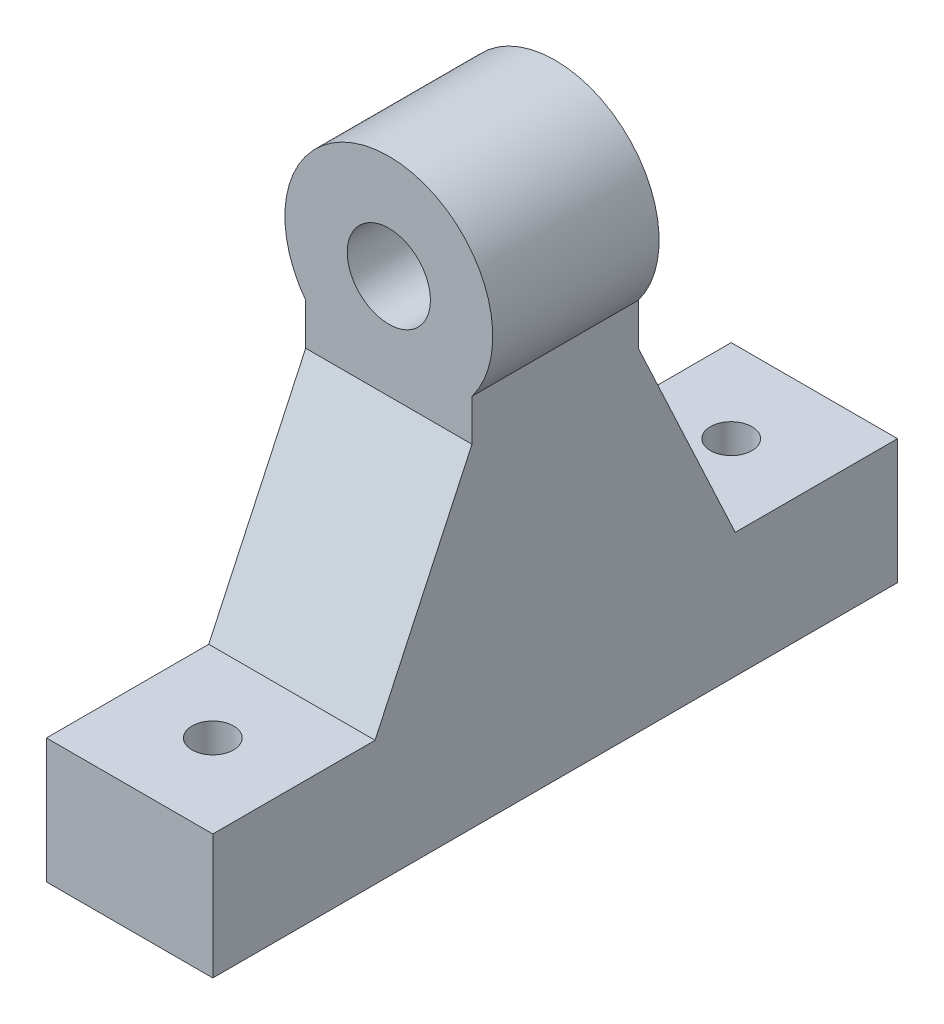
from build123d import *

# Parameters (mm, degrees)
SKETCH_1_R           = 12.5
SKETCH_1_R_2         = 5
EXTRUDE_1_DEPTH      = 10
EXTRUDE_3_DEPTH      = 10
EXTRUDE_4_REACH      = 60.746
EXTRUDE_4_END_RADIUS = 12.5
SKETCH_6_W           = 20
SKETCH_6_H           = 20
HOLE_WIZARD_M6_1_D   = 5


with BuildPart() as part:
    # 草图1 → 凸台-拉伸1 (new, symmetric)
    with BuildSketch(Plane.XY):
        Circle(SKETCH_1_R)
        Circle(SKETCH_1_R_2, mode=Mode.SUBTRACT)
    extrude(amount=EXTRUDE_1_DEPTH, both=True)



with BuildPart() as body_2:
    # 草图5 → 凸台-拉伸3 (new, symmetric)
    with BuildSketch(Plane(origin=(0, 0, 0), x_dir=(0, 0, -1), z_dir=(1, 0, 0))):
        Polygon((10, -12.5), (21.657691454, -37.5), (41.168402769, -37.5), (41.168402769, -52.5), (-41.168402769, -52.5), (-41.168402769, -37.5), (-21.657691454, -37.5), (-10, -12.5), align=None)
    extrude(amount=EXTRUDE_3_DEPTH, both=True)


with BuildPart() as part_1:
    add(part.part)

    add(body_2.part)  # 凸台-拉伸4 merges body 2
    # 凸台-拉伸4: up to this cylinder (the profile starts outside it)
    extrude_4_end = Plane(origin=(0, 0, 0), z_dir=(0, 0, -1)) * Cylinder(EXTRUDE_4_END_RADIUS, 147.492, mode=Mode.PRIVATE)
    # 草图6 → 凸台-拉伸4 (add, up to the surface)
    with BuildSketch(Plane(origin=(0, -12.5, 0), x_dir=(1, 0, 0), z_dir=(0, 1, 0)), mode=Mode.PRIVATE) as extrude_4_sk1:
        Rectangle(SKETCH_6_W, SKETCH_6_H)
    extrude_4_tool1 = extrude(extrude_4_sk1.sketch, amount=EXTRUDE_4_REACH, mode=Mode.PRIVATE) - extrude_4_end
    add(extrude_4_tool1.solids().sort_by_distance((0, -12.5, 0))[0])
    add(extrude_4_tool1.solids().sort_by_distance((0, -12.5, 0))[1])

    # M6 螺纹孔1 (through all)
    with Locations(Plane(origin=(0, -37.5, -31.168402769), x_dir=(0, 0, 1), z_dir=(0, 1, 0))):
        with Locations((0, 0)):
            hole_wizard_m6_1 = Hole(HOLE_WIZARD_M6_1_D / 2)

    # 镜向1: M6 螺纹孔1 across plane
    add(hole_wizard_m6_1.mirror(Plane.XY), mode=Mode.SUBTRACT)


solid = part_1.part
